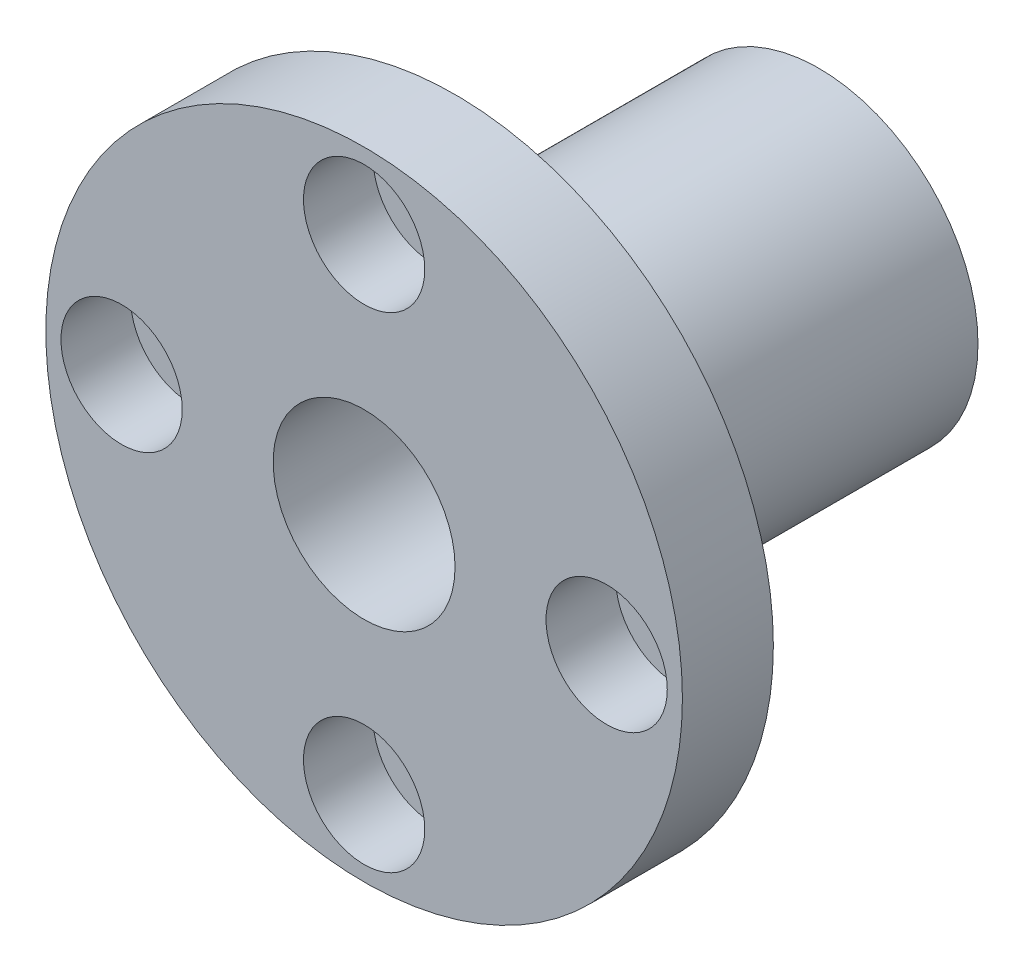
from build123d import *

# Parameters (mm, degrees)
SKETCH_1_R                = 10.5
SKETCH_1_R_2              = 6
EXTRUDE_1_DEPTH           = 15
SKETCH_2_R                = 21
SKETCH_2_R_2              = 10.5
EXTRUDE_2_DEPTH           = 6
HOLE_WIZARD_1_D           = 4.5
HOLE_WIZARD_1_DEPTH       = 11.5
HOLE_WIZARD_1_CBORE_D     = 8
HOLE_WIZARD_1_CBORE_DEPTH = 4.6
HOLE_WIZARD_1_TIP         = 1.351936393


with BuildPart() as part:
    # 草图1 → 凸台-拉伸1 (new, symmetric)
    with BuildSketch(Plane.XY):
        Circle(SKETCH_1_R)
        Circle(SKETCH_1_R_2, mode=Mode.SUBTRACT)
    extrude(amount=EXTRUDE_1_DEPTH, both=True)

    # 草图2 → 凸台-拉伸2 (add)
    with BuildSketch(Plane.XY.offset(15)):
        Circle(SKETCH_2_R)
        Circle(SKETCH_2_R_2, mode=Mode.SUBTRACT)
    extrude(amount=-EXTRUDE_2_DEPTH)

    # 打孔尺寸(%根据)内六角圆柱头螺钉的类型1
    with Locations(Plane.XY.offset(15)):
        with Locations((0, 16), (16, 0), (0, -16), (-16, 0)):
            CounterBoreHole(HOLE_WIZARD_1_D / 2, HOLE_WIZARD_1_CBORE_D / 2, HOLE_WIZARD_1_CBORE_DEPTH, depth=HOLE_WIZARD_1_DEPTH)
            with Locations((0, 0, -(HOLE_WIZARD_1_DEPTH + HOLE_WIZARD_1_TIP / 2))):  # 118° drill point
                Cone(0, HOLE_WIZARD_1_D / 2, HOLE_WIZARD_1_TIP, mode=Mode.SUBTRACT)


solid = part.part
